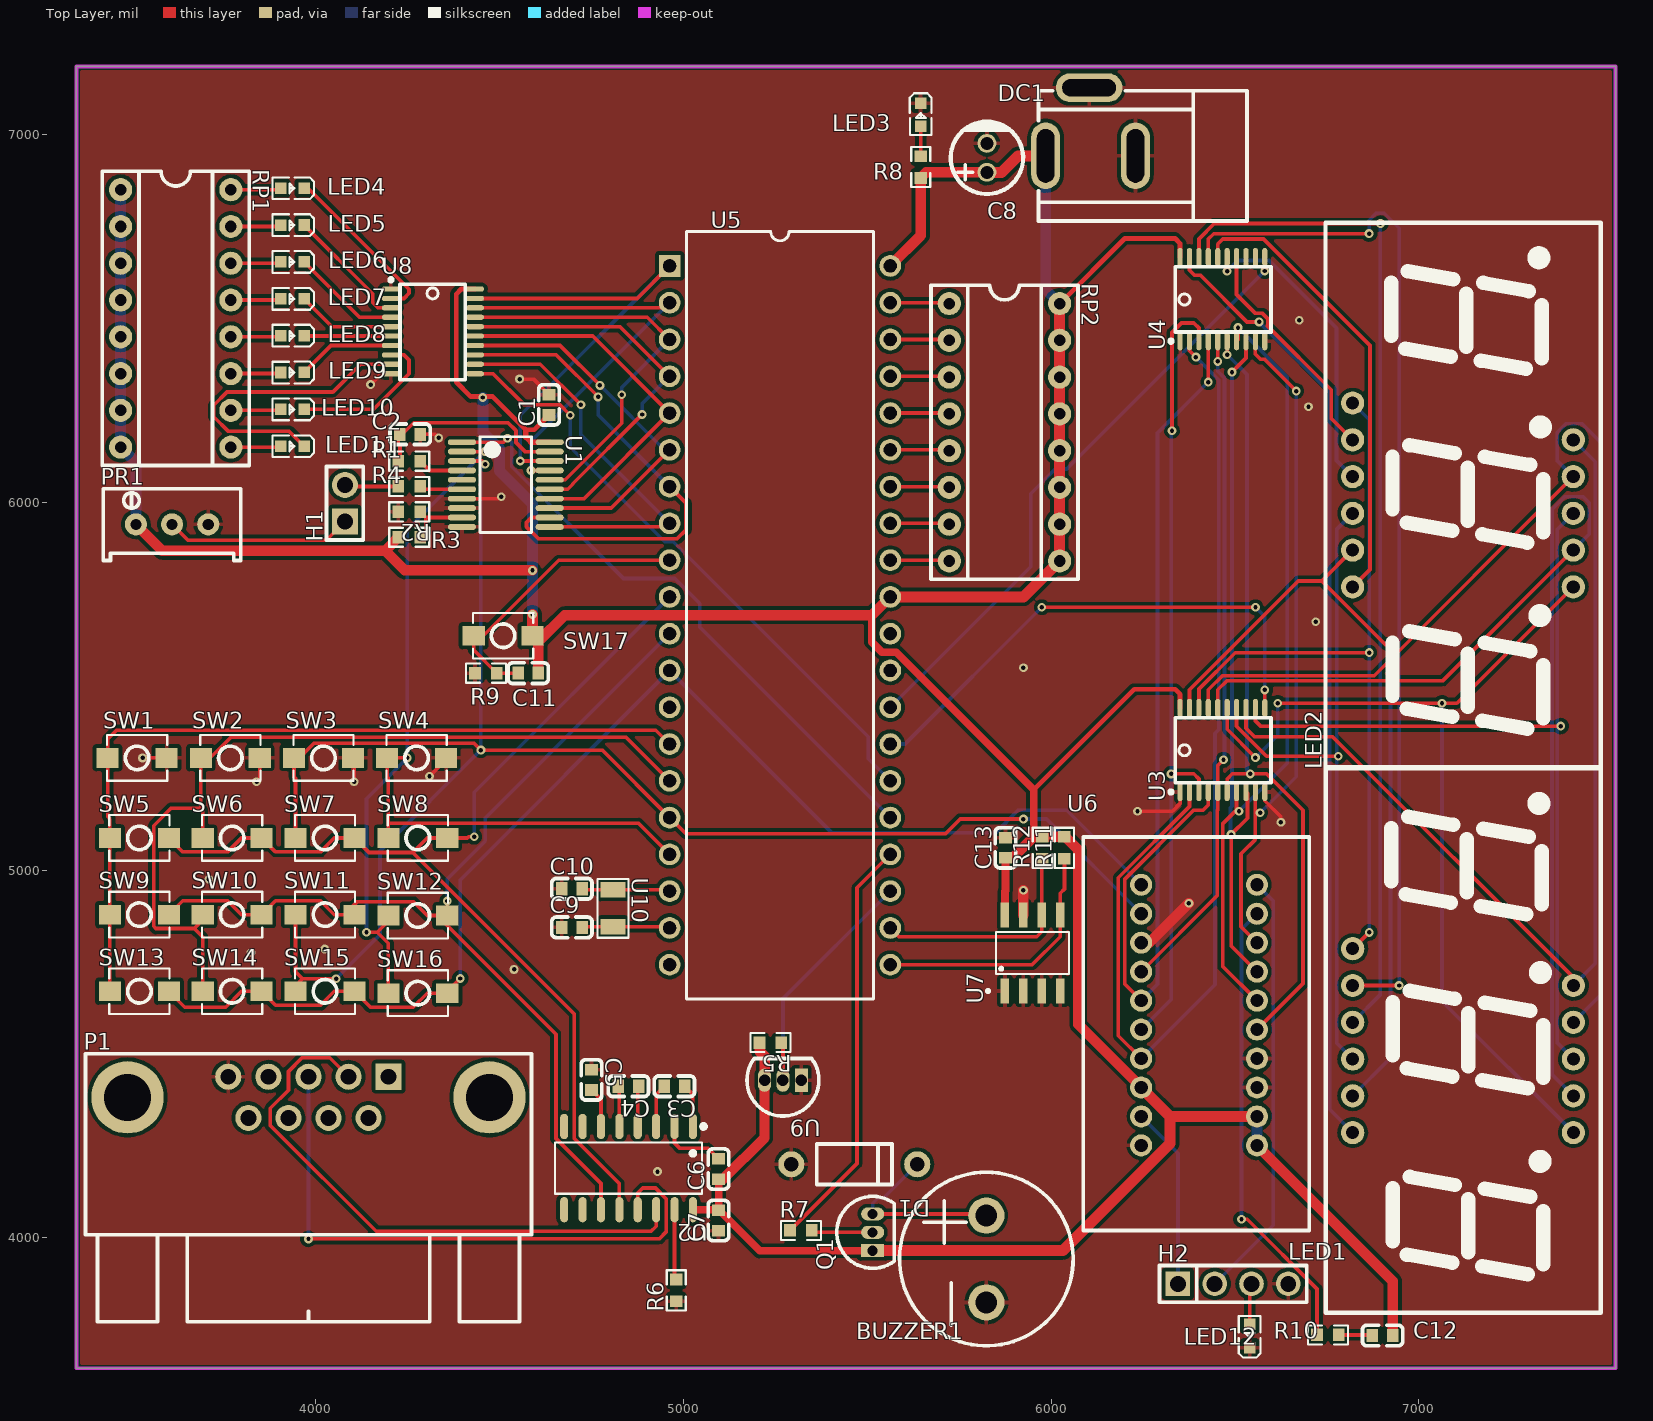
[diagram p0: Top Layer view]
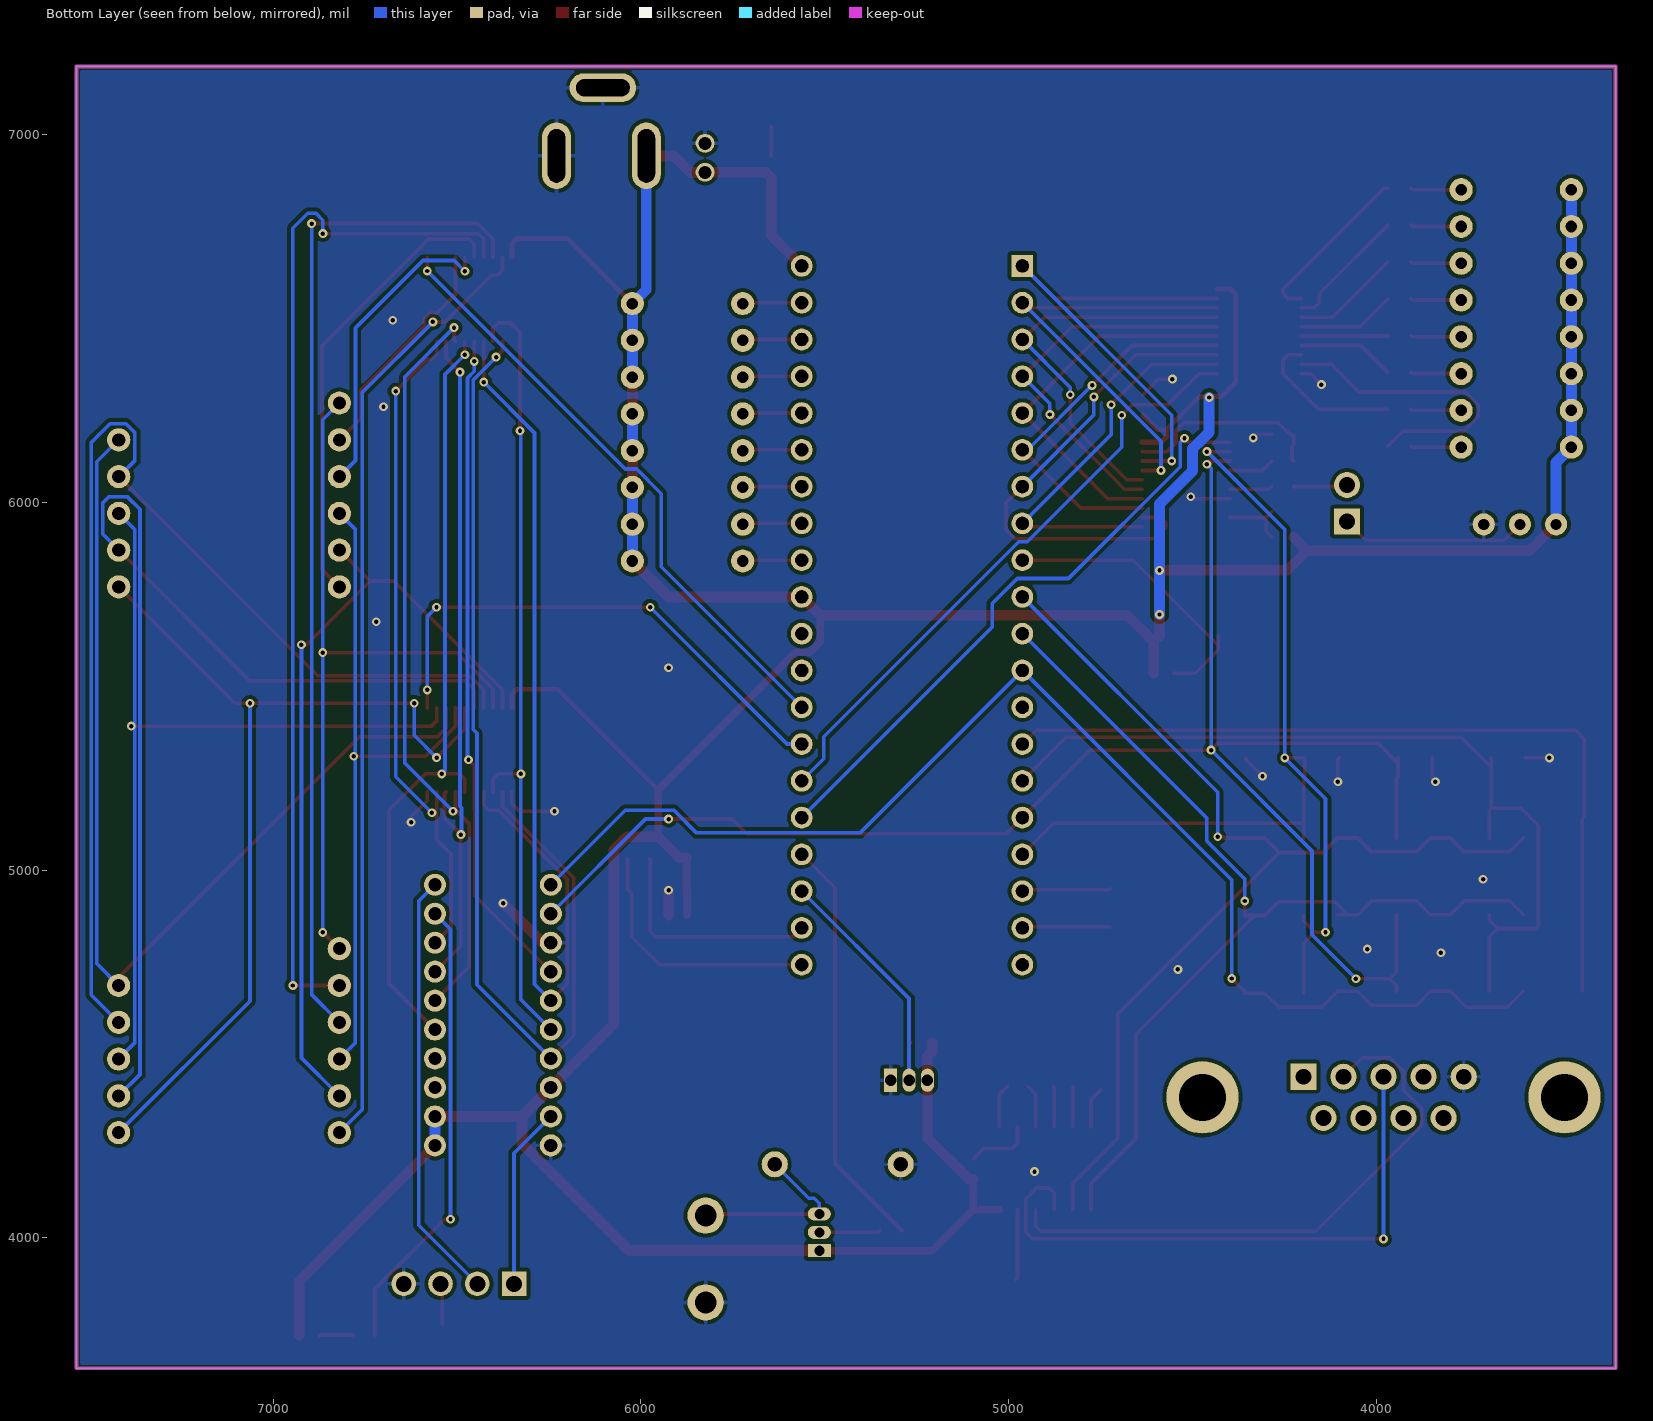
[diagram p1: Bottom Layer view, seen from below]
# Altium PCB MISC51981.pcbdoc
Units mil, origin at the board's own origin, x right, y up, seen from the top; angles counter-clockwise.
Board outline 4185 x 3540 mil, 2 copper layers (Top Layer, Bottom Layer), stack 62.206 mil thick; 74 components, 100 nets, 357 pads, 76 vias.

## Layer stack, top to bottom
Top Solder Mask Layer: solder mask 0.394, Dk 3.3
Top Layer: signal copper 1.379
Dielectric1: surface 59.449, FR4, Dk 4.5
Bottom Layer: signal copper 1.378
Bottom Solder Mask Layer: solder mask 0.394, Dk 3.3

## Board outline
3350,7185 3350,3645 7535,3645 7535,7185

## Design rules (kind name [scope] priority, off if disabled: settings)
BoardOutlineClearance copperThickness2oz_1 [All] p2 off: genericclearance=7.99 ignorepadtopadclearanceinfootprint=FALSE except(0: Arc-SplitContinuation Track-SplitContinuation SMDPad-SplitContinuation THPad-SplitContinuation Via-SplitContinuation Fill-SplitContinuation Region-SplitContinuation Poly-SplitContinuation Text-SplitContinuation Hole-SplitContinuation; 5.98: Arc-CutoutEdge SMDPad-CutoutEdge THPad-CutoutEdge Via-CutoutEdge Fill-CutoutEdge Region-CutoutEdge Text-CutoutEdge; 6.93: Hole-OutlineEdge Hole-CutoutEdge; 10: Poly-OutlineEdge Poly-CutoutEdge; 11.81: Arc-OutlineEdge Track-OutlineEdge SMDPad-OutlineEdge THPad-OutlineEdge Via-OutlineEdge Fill-OutlineEdge Region-OutlineEdge Text-OutlineEdge Track-CutoutEdge)
BoardOutlineClearance copperThickness1oz_1 [All] p4: genericclearance=4.02 ignorepadtopadclearanceinfootprint=FALSE except(0: Arc-SplitContinuation Track-SplitContinuation SMDPad-SplitContinuation THPad-SplitContinuation Via-SplitContinuation Fill-SplitContinuation Region-SplitContinuation Poly-SplitContinuation Text-SplitContinuation Hole-SplitContinuation; 6: SMDPad-CutoutEdge THPad-CutoutEdge Via-CutoutEdge Fill-CutoutEdge Region-CutoutEdge Text-CutoutEdge; 6.93: Hole-OutlineEdge Hole-CutoutEdge; 10: Poly-OutlineEdge Poly-CutoutEdge; 11.8: Arc-OutlineEdge Track-OutlineEdge SMDPad-OutlineEdge THPad-OutlineEdge Via-OutlineEdge Fill-OutlineEdge Region-OutlineEdge Text-OutlineEdge; 11.81: Arc-CutoutEdge Track-CutoutEdge)
Clearance copperThickness2oz [All] p1 off: gap=7.99 ignorepadtopadclearanceinfootprint=FALSE except(5.98: SMDPad-Track SMDPad-SMDPad THPad-Track SMDPad-THPad THPad-THPad Track-Via SMDPad-Via THPad-Via Via-Via Fill-Track Region-Track Fill-SMDPad Region-SMDPad Fill-THPad Region-THPad Fill-Via Region-Via Fill-Fill Fill-Region Region-Region Arc-Track Arc-SMDPad Arc-THPad Arc-Via Fill-Arc Region-Arc Arc-Arc Text-Track SMDPad-Text Text-THPad Text-Via Fill-Text Region-Text Arc-Text Text-Text; 6.93: Hole-Track Hole-SMDPad Hole-THPad Hole-Via Fill-Hole Region-Hole Hole-Arc Hole-Text; 10: Poly-Track Poly-SMDPad Poly-THPad Poly-Via Poly-Fill Poly-Region Poly-Poly Poly-Arc Poly-Text Poly-Hole)
Clearance copperThickness1oz [All] p3: gap=4.02 ignorepadtopadclearanceinfootprint=FALSE except(5.98: SMDPad-Track SMDPad-SMDPad THPad-Track SMDPad-THPad THPad-THPad Track-Via SMDPad-Via THPad-Via Via-Via Fill-Track Region-Track Fill-SMDPad Region-SMDPad Fill-THPad Region-THPad Fill-Via Region-Via Fill-Fill Fill-Region Region-Region; 6: Arc-Track Arc-SMDPad Arc-THPad Arc-Via Fill-Arc Region-Arc Arc-Arc Text-Track SMDPad-Text Text-THPad Text-Via Fill-Text Region-Text Arc-Text Text-Text; 6.93: Hole-Track Hole-SMDPad Hole-THPad Hole-Via Fill-Hole Region-Hole Hole-Arc Hole-Text; 10: Poly-Track Poly-SMDPad Poly-THPad Poly-Via Poly-Fill Poly-Region Poly-Poly Poly-Arc Poly-Text Poly-Hole)
Creepage creepage [All] p1: checkdistance=0 ignoreinternallayers=TRUE applytopolygonpour=TRUE
DiffPairsRouting differentialPair [All] p1: maxlimit=6 minlimit=6 mostfreqgap=6 toplayer_minwidth=5 toplayer_prefwidth=10 toplayer_maxwidth=100 toplayer_mingap=6 toplayer_prefgap=6 toplayer_maxgap=6 bottomlayer_minwidth=5 bottomlayer_prefwidth=10 bottomlayer_maxwidth=100 bottomlayer_mingap=6 bottomlayer_prefgap=6 bottomlayer_maxgap=6 maxuncoupledlength=10
HoleToHoleClearance otherClearance [All] p1: gap=11.81 allowstackedmicrovias=TRUE
Length netLength [All] p1: minlimit=0 maxlimit=0
MatchedLengths netLengthTolerance [All] p1: tolerance=1000
PasteMaskExpansion pasteMaskExpansion [All] p1: expansion=0
PlaneConnect innerPlane [All] p1: planeconnectstyle=Relief reliefexpansion=20 reliefentries=4 reliefconductorwidth=10 reliefairgap=10
PolygonConnect copperRegion [All] p1: connectstyle=Relief reliefconductorwidth=10 reliefentries=4 polygonreliefangle="90 Angle" airgapwidth=10 via.connectstyle=Relief via.reliefconductorwidth=10 via.reliefentries=4 via.polygonreliefangle="90 Angle" via.airgapwidth=10
RoutingVias viaSize [All] p1: holewidth=12.01 width=24.02 viastyle="Through Hole" minholewidth=11.81 minwidth=19.68 maxholewidth=248.03 maxwidth=393.7
SolderMaskExpansion solderMaskExpansion [IsVia] p1: expansion=-1000 istentingtop=TRUE
SolderMaskExpansion solderMaskExpansion [All] p2: expansion=2 istentingtop=FALSE
Width copperThickness2oz_2 [All] p1 off: maxlimit=100 minlimit=8 preferedwidth=10
Width PWR [(InNet('VCC'))] p2: maxlimit=10 minlimit=10 preferedwidth=10 toplayer_minwidth=10 toplayer_maxwidth=100 toplayer_prefwidth=30 bottomlayer_minwidth=10 bottomlayer_maxwidth=100 bottomlayer_prefwidth=30
Width copperThickness1oz_2 [All] p3: maxlimit=10 minlimit=10 preferedwidth=10 toplayer_minwidth=10 toplayer_maxwidth=100 toplayer_prefwidth=10 bottomlayer_minwidth=10 bottomlayer_maxwidth=100 bottomlayer_prefwidth=10

## Components (designator, comment, footprint, x,y, rotation, side; value= is the part's Value field where it differs from the comment)
BUZZER1 "buzzer" BUZ-TH_BD12.0-P6.00-D0.9-RD 5824.07,3942.5 r90 top
C1 "104" C0603 4635,6265 r90 top
C2 "104" C0603 4257.19,6185 r0 top
C3 "104" C0603 4975.96,4412.17 r180 top
C4 "104" C0603 4850.96,4412.17 r180 top
C5 "104" C0603 4750.56,4429.6 r270 top
C6 "104" C0603 5095.96,4187.17 r90 top
C7 "104" C0603 5095.96,4047.17 r90 top
C8 "100uF" CAP-TH_BD5.0-P2.00-D0.8-FD-10UF50VC110GL 5825.71,6936.62 r90 top
C9 "20PF" C0603 4697.26,4844.24 r0 top
C10 "20PF" C0603 4697.26,4949.24 r0 top
C11 "10uF" C0603 4578.45,5535.44 r0 top
C12 "104" C0603 6901.47,3734.39 r0 top
C13 "104" C0603 5876.39,5060.56 r90 top
D1 "" DO_1N4007 5465,4200 r180 top
DC1 "" DC-005_2.5 6112.46,6954.71 r0 top
H1 "" HDR-TH_2P-P2.54-V-M-1 4080,5997.34 r90 top
H2 "" HDR-TH_4P-P2.54-V-M 6495,3875 r0 top
LED1 "3631BS" LED-SEG-TH_11P-L37.5-W19.0-P2.54-LS15.2-BL_1 7120.32,4536.17 r90 top
LED2 "3631BS" LED-SEG-TH_11P-L37.5-W19.0-P2.54-LS15.2-BL_1 7120,6020 r90 top
LED3 "" LED_0603 5645.71,7051.62 r270 top
LED4 "" LED_0603 3935.58,6853.85 r180 top
LED5 "" LED_0603 3935.58,6753.63 r180 top
LED6 "" LED_0603 3935.58,6653.41 r180 top
LED7 "" LED_0603 3935.58,6553.19 r180 top
LED8 "" LED_0603 3935.58,6452.98 r180 top
LED9 "" LED_0603 3935.58,6352.76 r180 top
LED10 "" LED_0603 3935.58,6252.54 r180 top
LED11 "" LED_0603 3935.58,6152.32 r180 top
LED12 "" LED_0603 6540,3735 r90 top
P1 "DB9FL" DB9-TH_DB9F 3980.96,4382.17 r0 top
PR1 "10kΩ" R_3296 3610,5945 r0 top
Q1 "" S8550P_TO-92 5515,4015 r90 top
R1 "10K" R0603 4255,6112.04 r0 top
R2 "1K" R0603 4255,5974.01 r180 top
R3 "1K" R0603 4255,5905 r0 top
R4 "510K" R0603 4255,6043.03 r0 top
R5 "4.7K" R0603 5237.02,4531.02 r180 top
R6 "0" R0603 4980.96,3857.17 r90 top
R7 "2K" R0603 5320,4020 r0 top
R8 "1K" R0603 5645.71,6911.62 r270 top
R9 "10K" R0603 4463.45,5535.44 r0 top
R10 "0" R0603 6752.91,3736.03 r0 top
R11 "4.7K" R0603 6036.39,5060.56 r90 top
R12 "4.7K" R0603 5976.39,5060.56 r90 top
RP1 "" DIP-16_L20.3-W10.2-P2.54-LS7.6-BL 3620,6500 r270 top
RP2 "" DIP-16_L20.3-W10.2-P2.54-LS7.6-BL 5873.45,6190.44 r270 top
SW1 "" Key_SMD_3x4x2 3515,5305 r180 top
SW2 "" Key_SMD_3x4x2 3768.33,5305 r180 top
SW3 "" Key_SMD_3x4x2 4021.67,5305 r180 top
SW4 "" Key_SMD_3x4x2 4275,5305 r180 top
SW5 "" Key_SMD_3x4x2 3521.09,5087.32 r0 top
SW6 "" Key_SMD_3x4x2 3773.46,5087.32 r0 top
SW7 "" Key_SMD_3x4x2 4025.84,5087.32 r0 top
SW8 "" Key_SMD_3x4x2 4278.21,5087.32 r0 top
SW9 "" Key_SMD_3x4x2 3521.09,4878.83 r0 top
SW10 "" Key_SMD_3x4x2 3773.46,4878.83 r0 top
SW11 "" Key_SMD_3x4x2 4025.84,4878.83 r0 top
SW12 "" Key_SMD_3x4x2 4278.21,4876.33 r0 top
SW13 "" Key_SMD_3x4x2 3521.09,4670.34 r0 top
SW14 "" Key_SMD_3x4x2 3773.46,4670.34 r0 top
SW15 "" Key_SMD_3x4x2 4025.84,4670.34 r0 top
SW16 "" Key_SMD_3x4x2 4278.21,4665.34 r0 top
SW17 "" Key_SMD_3x4x2 4510.24,5637.16 r180 top
U1 "ADC0804CN" ADC0804CN 4529.5,6063.27 r270 top
U2 "MAX232ESE" MAX232ESE 5055.96,4302.17 r180 top
U3 "MC74HC573DW" MC74HC573DW 6350.95,5212.39 r90 top
U4 "MC74HC573DW" MC74HC573DW 6350.95,6438.19 r90 top
U5 "P89C51RC2HBP" P89C51RC23N_01 5218.38,5544.96 r270 top
U6 "DAC0832LCJ" DAC0832LCJ 6560,4960 r0 top
U7 "AT24C02" SOIC-8_L5.0-W4.0-P1.27-LS6.2-TL 5949.75,4774.49 r90 top
U8 "MC74HC573DW" MC74HC573DW 4205,6580 r0 top
U9 "DS18B20" TO-92-3_L4.9-W3.7-P1.27-L 5271.01,4428.68 r180 top
U10 "32768/10ppm/12.5pF" osc-smd_l3.2-w1.5 4808.9,4896.03 r270 top

## Footprints (in the part's own frame and the unit in brackets; to place one, negate y for a bottom-side part, rotate by r counter-clockwise, add the part's x,y. Pads: shape width x height; smd on the part's side, far side on the other; paste and mask are expansions set on the pad)
ADC0804CN [mm]
  oval 0.4x1.95 smd: 1(-2.544,-3.334) 2(-1.894,-3.334) 3(-1.244,-3.334) 4(-0.594,-3.334) 5(0.056,-3.334) 6(0.706,-3.334) 7(1.356,-3.334) 8(2.006,-3.334) 9(2.656,-3.334) 10(3.306,-3.334) 11(3.306,2.724) 12(2.656,2.724) 13(2.006,2.724) 14(1.356,2.724) 15(0.706,2.724) 16(0.056,2.724) 17(-0.594,2.724) 18(-1.244,2.724) 19(-1.894,2.724) 20(-2.544,2.724)
  silkscreen extent -2.92,-2.08 3.68,1.47
BUZ-TH_BD12.0-P6.00-D0.9-RD [mm]
  round 2.5 hole 1.5 paste+0 mask+0.05: 1(-3,0) 2(3,0)
  silkscreen extent -5.99,-5.99 5.99,5.99
C0603 [mm]
  rect 0.8x0.9 smd: 1(-0.7,0) 2(0.7,0)
  silkscreen extent -1.39,-0.71 1.39,0.71
CAP-TH_BD5.0-P2.00-D0.8-FD-10UF50VC110GL [mm]
  round 1.3 hole 0.9 paste+0 mask+0.051: 1(-1,0) 2(1,0)
  silkscreen extent -2.5,-2.5 2.5,2.5
DAC0832LCJ [mil]
  round 60 hole 36 paste+0 mask+2: 1(-314.96,0) 2(-314.96,-78.74) 3(-314.96,-157.48) 4(-314.96,-236.22) 5(-314.96,-314.96) 6(-314.96,-393.7) 7(-314.96,-472.44) 8(-314.96,-551.18) 9(-314.96,-629.92) 10(-314.96,-708.66) 11(0,0) 12(0,-78.74) 13(0,-157.48) 14(0,-236.22) 15(0,-314.96) 16(0,-393.7) 17(0,-472.44) 18(0,-551.18) 19(0,-629.92) 20(0,-708.66)
  silkscreen extent -472,-940 142,130
DB9-TH_DB9F [mm]
  rect 1.8x1.8 hole 1.1: 1(5.54,1.42)
  round 1.8 hole 1.1: 2(2.77,1.42) 3(0,1.42) 4(-2.77,1.42) 5(-5.54,1.42) 6(4.155,-1.42) 7(1.385,-1.42) 8(-1.385,-1.42) 9(-4.155,-1.42)
  round 5 hole 3.25: 10(-12.5,0) 11(12.5,0)
  silkscreen extent -15.4,-15.5 15.4,3
DC-005_2.5 [mm]
  oval 2x4.6 hole 1.2 slot 3.7 at 90 deg paste+0 mask+0.051: 1(-3.227,-0.318) 2(2.973,-0.318)
  oval 4.6x2 hole 1.2 slot 3.7 at 0 deg paste+0 mask+0.051: 3(-0.227,4.382)
  silkscreen extent -3.73,-4.82 10.67,4.18
DIP-16_L20.3-W10.2-P2.54-LS7.6-BL [mm]
  round 1.6 hole 0.8: 1(-8.89,-3.81) 2(-6.35,-3.81) 3(-3.81,-3.81) 4(-1.27,-3.81) 5(1.27,-3.81) 6(3.81,-3.81) 7(6.35,-3.81) 8(8.89,-3.81) 9(8.89,3.81) 10(6.35,3.81) 11(3.81,3.81) 12(1.27,3.81) 13(-1.27,3.81) 14(-3.81,3.81) 15(-6.35,3.81) 16(-8.89,3.81)
  silkscreen extent -10.16,-5.08 10.16,5.08
DO_1N4007 [mm]
  round 1.8 hole 1 paste+0 mask+0.051: 1(-4.35,0) 2(4.35,0)
  silkscreen extent -2.6,-1.4 2.6,1.4
HDR-TH_2P-P2.54-V-M-1 [mm]
  rect 1.8x1.8 hole 1.1: 1(-1.27,0)
  round 1.8 hole 1.1: 2(1.27,0)
  silkscreen extent -2.54,-1.27 2.54,1.27
HDR-TH_4P-P2.54-V-M [mm]
  rect 1.7x1.7 hole 1.1: 1(-3.81,0)
  round 1.7 hole 1.1: 2(-1.27,0) 3(1.27,0) 4(3.81,0)
  silkscreen extent -5.08,-1.27 5.08,1.27
Key_SMD_3x4x2 [mm]
  rect 1.53x1.36 smd paste+0 mask+0.051: 1(-2.035,0) 2(2.035,0)
  silkscreen extent -2.08,-1.58 2.08,1.58
LED-SEG-TH_11P-L37.5-W19.0-P2.54-LS15.2-BL_1 [mm]
  round 1.6 hole 0.9: 1(-6.35,-7.62) 2(-3.81,-7.62) 3(-1.27,-7.62) 4(1.27,-7.62) 5(3.81,-7.62) 7(6.35,7.62) 8(3.81,7.62) 9(1.27,7.62) 10(-1.27,7.62) 11(-3.81,7.62) 12(-6.35,7.62)
  silkscreen extent -18.8,-9.51 18.8,9.49
LED_0603 [mil]
  rect 31.5x31.5 smd paste+0 mask+2: 1(-33.5,-0.4) 2(29.5,-0.2)
  silkscreen extent -61,-30 53,30
MAX232ESE [mm]
  oval 0.56x1.745 smd paste+0.102 mask+0.051: 1(0.755,-0.016) 2(2.025,-0.016) 3(3.295,-0.016) 4(4.565,-0.016) 5(5.835,-0.016) 6(7.105,-0.016) 7(8.375,-0.016) 8(9.645,-0.016) 9(9.645,5.728) 10(8.375,5.728) 11(7.105,5.728) 12(5.835,5.728) 13(4.565,5.728) 14(3.295,5.728) 15(2.025,5.728) 16(0.755,5.728)
  silkscreen extent -0.13,-0.17 10.28,4.63
MC74HC573DW [mm]
  oval 1.26x0.36 smd: 1(0,0) 2(0,-0.65) 3(0,-1.3) 4(0,-1.95) 5(0,-2.6) 6(0,-3.25) 7(0,-3.9) 8(0,-4.55) 9(0,-5.2) 10(0,-5.85) 11(5.8,-5.85) 12(5.8,-5.2) 13(5.8,-4.55) 14(5.8,-3.9) 15(5.8,-3.25) 16(5.8,-2.6) 17(5.8,-1.95) 18(5.8,-1.3) 19(5.8,-0.65) 20(5.8,0)
  silkscreen extent -0.05,-6.27 5.13,0.68
osc-smd_l3.2-w1.5 [mm]
  rect 1.05x1.7 smd: 1(-1.275,0) 2(1.275,0)
  silkscreen extent -2.03,-1.08 2.03,1.08
P89C51RC23N_01 [mm]
  rect 1.5x1.5 hole 0.9 slot 0.905 at 90 deg paste+0 mask+0.051: 1(-27.883,-6.489)
  round 1.5 hole 0.9 slot 0.905 at 90 deg paste+0 mask+0.051: 2(-25.343,-6.489) 3(-22.803,-6.489) 4(-20.263,-6.489) 5(-17.723,-6.489) 6(-15.183,-6.489) 7(-12.643,-6.489) 8(-10.103,-6.489) 9(-7.563,-6.489) 10(-5.023,-6.489) 11(-2.483,-6.489) 12(0.057,-6.489) 13(2.597,-6.489) 14(5.137,-6.489) 15(7.677,-6.489) 16(10.217,-6.489) 17(12.757,-6.489) 18(15.297,-6.489) 19(17.837,-6.489) 20(20.377,-6.489) 21(20.377,8.751) 22(17.837,8.751) 23(15.297,8.751) 24(12.757,8.751) 25(10.217,8.751) 26(7.677,8.751) 27(5.137,8.751) 28(2.597,8.751) 29(0.057,8.751) 30(-2.483,8.751) 31(-5.023,8.751) 32(-7.563,8.751) 33(-10.103,8.751) 34(-12.643,8.751) 35(-15.183,8.751) 36(-17.723,8.751) 37(-20.263,8.751) 38(-22.803,8.751) 39(-25.343,8.751) 40(-27.883,8.751)
  silkscreen extent -30.25,-5.32 22.75,7.58
R0603 [mil]
  rect 31.75x34.02 smd paste-3937.01 mask+2: 1(-29.66,0) 2(29.66,0)
  silkscreen extent -55,-26 55,26
R_3296 [mil]
  round 60 hole 30 paste+0 mask+2: 1(-98.4,-5) 2(0,-5) 3(98.4,-5)
  silkscreen extent -187,-103 187,92
S8550P_TO-92 [mm]
  rect 0.9x1.6 hole 0.7 paste+0 mask+0.051: 1(-1.27,0)
  oval 0.9x1.6 hole 0.7 paste+0 mask+0.051: 2(0,0) 3(1.27,0)
  silkscreen extent -2.48,-1.5 2.48,2.48
SOIC-8_L5.0-W4.0-P1.27-LS6.2-TL [mil]
  rect 68.92x23.18 smd: 1(-103.36,75) 2(-103.36,25) 3(-103.36,-25) 4(-103.36,-75) 5(103.36,-75) 6(103.36,-25) 7(103.36,25) 8(103.36,75)
  silkscreen extent -107,-99 57,125
TO-92-3_L4.9-W3.7-P1.27-L [mm]
  rect 0.9x1.6 hole 0.8: 1(-1.27,0)
  oval 0.9x1.6 hole 0.8: 2(0,0) 3(1.27,0)
  silkscreen extent -2.48,-1.5 2.48,2.48

## Via types
v1: diameter 24.02, hole 12, Top Layer to Bottom Layer, 76 vias

## Nets (pads, with @x,y where several pads share a name; then routed paths per layer and width w, separated by ;. In a path a pad name is that pad's centre, name@x,y a point inside that pad or via, vN(x,y) a via of type N, cw(c..) or ccw(c..) an arc to the next point about the centre after c; other vN are vias at no path point)
18B20: R5.1 U5.23 U9.2 | length 739.1
  Top Layer w10: R5.1 5271.01,4526.69 U9.2
  Bottom Layer w10: U9.2 5271.01,4650.81 U5.23
$1N14: R1.2 U1.4 | length 124.1
  Top Layer w10: R1.2 4310.04,6086.66 U1.4@4398.25,6086.66
$1N15: C2.1 R1.1 U1.19 | length 558.8
  Top Layer w10: R1.1 4229.93,6116.63 4229.93,6151.61 4225.34,6156.2 C2.1@4225.34,6174.83 ; C2.1 4225.34,6180.71 C2.1@4225.34,6174.83 ; U1.19@4636.75,6137.84 4569.86,6137.84 4545,6162.7 4545,6195 4523.4,6216.6 4267.11,6216.6 C2.1@4225.34,6174.83
$1N18: H1.1 PR1.2 | length 509
  Top Layer w10: PR1.2 3653.36,5896.64 4029.3,5896.64 H1.1
$1N20: R2.1 R3.2 U1.9 | length 180
  Top Layer w10: R3.2 4299.98,5920.32 R2.1@4299.98,5958.7 ; R2.1 R2.1@4299.98,5958.7 ; U1.9@4398.25,5958.7 R2.1@4299.98,5958.7
$1N23: R4.2 U1.6 | length 116.7
  Top Layer w10: R4.2 4292.22,6035.47 U1.6@4398.25,6035.47
$1N24: H1.2 R4.1 | length 147.1
  Top Layer w10: H1.2 4084.31,6043.03 R4.1
$1N28: C3.1 U2.1 | length 118.8
  Top Layer w10: C3.1 5026.22,4389.46 U2.1
$1N29: C3.2 U2.3 | length 118.5
  Top Layer w10: U2.3 4926.22,4389.98 C3.2
$1N30: C4.2 U2.5 | length 110.5
  Top Layer w10: C4.2 4826.22,4409.34 U2.5
$1N31: C4.1 U2.4 | length 110.3
  Top Layer w10: U2.4 4876.22,4409.86 C4.1
$1N34: R6.2 U2.15 | length 191.8
  Top Layer w10: U2.15 4976.22,3891.56 R6.2
$1N36: P1.3 U2.13 | length 1651.5
  Top Layer w10: v1(3980.96,3997.14) 4934.41,3997.14 4953.36,4016.09 4953.36,4106.56 4924.44,4135.48 4889.99,4135.48 4876.22,4121.71 U2.13
  Bottom Layer w10: v1(3980.96,3997.14) P1.3
$1N37: P1.2 U2.14 | length 1586.6
  Top Layer w10: P1.2 4038.48,4489.61 3963.45,4489.61 3926.43,4452.59 3926.43,4401.4 3877.24,4352.21 3877.24,4305.64 4165.1,4017.78 4912.45,4017.78 4926.22,4031.55 U2.14
$1N38: C5.2 U2.6 | length 109.9
  Top Layer w10: C5.2 4776.22,4376.38 U2.6
$1N40: C6.2 U2.2 | length 182.6
  Top Layer w10: U2.2 4976.22,4257.73 4989.99,4243.96 5066.72,4243.96 C6.2
$1N109: BUZZER1.2 D1.1 Q1.3 | length 505
  Top Layer w10: Q1.3 5819.68,4065 BUZZER1.2
  Bottom Layer w10: Q1.3 5515,4093.95 5528.77,4107.72 5543.98,4107.72 D1.1
$1N111: Q1.2 R7.2 | length 167.4
  Top Layer w10: R7.2 5354.66,4015 Q1.2
$1N114: LED3.2 R8.1 | length 80.9
  Top Layer w10: LED3.2 5645.51,6941.48 R8.1
$1N128: LED4.1 U8.2 | length 465.3
  Top Layer w10: LED4.1@3969.08,6854.25 3979.44,6854.25 4254.3,6579.39 4254.3,6568.18 4240.53,6554.41 U8.2
$1N129: LED5.1 U8.3 | length 343.7
  Top Layer w10: LED5.1 4155.7,6567.41 4155.7,6542.59 4169.47,6528.82 U8.3
$1N130: LED5.2 RP1.15 | length 137.7
  Top Layer w10: RP1.15 3902.25,6750 LED5.2
$1N131: LED7.2 RP1.13 | length 137.5
  Top Layer w10: RP1.13 3902.68,6550 LED7.2
$1N132: LED7.1 U8.5 | length 267.4
  Top Layer w10: LED7.1 4045.04,6477.64 U8.5
$1N133: LED6.1 U8.4 | length 298.3
  Top Layer w10: LED6.1 4119.67,6503.23 U8.4
$1N134: LED9.2 RP1.11 | length 137.3
  Top Layer w10: RP1.11 3903.12,6350 LED9.2
$1N135: LED9.1 U8.7 | length 266.3
  Top Layer w10: LED9.1 4042.38,6426.46 U8.7
$1N136: LED8.1 U8.6 | length 236.5
  Top Layer w10: LED8.1 3970.41,6452.05 U8.6
$1N137: LED11.2 RP1.9 | length 137.1
  Top Layer w10: RP1.9 3903.56,6150 LED11.2
$1N138: LED11.1 U8.9 | length 837.8
  Top Layer w10: LED11.1 3928.94,6192.86 3763.36,6192.86 3723.25,6232.97 3723.25,6263.68 3759.57,6300 4047.27,6300 4122.55,6375.28 U8.9
$1N139: LED10.1 U8.8 | length 417.9
  Top Layer w10: LED10.1 4157.9,6252.94 4254.3,6349.34 4254.3,6387.1 4240.53,6400.87 U8.8
$1N140: LED4.2 RP1.16 | length 137.8
  Top Layer w10: RP1.16 3902.03,6850 LED4.2@3906.08,6854.05
$1N141: LED6.2 RP1.14 | length 137.6
  Top Layer w10: RP1.14 3902.46,6650 LED6.2
$1N142: LED8.2 RP1.12 | length 137.4
  Top Layer w10: RP1.12 3902.9,6450 LED8.2
$1N143: LED10.2 RP1.10 | length 137.2
  Top Layer w10: RP1.10 3903.34,6250 LED10.2
$1N162: RP2.8 U5.32 | length 161.5
  Top Layer w10: U5.32 5721.17,5842.72 RP2.8
$1N163: RP2.7 U5.33 | length 161.5
  Top Layer w10: U5.33 5721.17,5942.72 RP2.7
$1N164: RP2.6 U5.34 | length 161.5
  Top Layer w10: U5.34 5721.17,6042.72 RP2.6
$1N165: RP2.5 U5.35 | length 161.5
  Top Layer w10: U5.35 5721.17,6142.72 RP2.5
$1N166: RP2.4 U5.36 | length 161.5
  Top Layer w10: U5.36 5721.17,6242.72 RP2.4
$1N167: RP2.3 U5.37 | length 161.5
  Top Layer w10: U5.37 5721.17,6342.72 RP2.3
$1N168: RP2.2 U5.38 | length 161.5
  Top Layer w10: U5.38 5721.17,6442.72 RP2.2
$1N169: RP2.1 U5.39 | length 161.5
  Top Layer w10: U5.39 5721.17,6542.72 RP2.1
$1N205: C12.1 R10.2 | length 92
  Top Layer w10: R10.2 6872.27,3736.03 C12.1
$1N206: R10.1 U6.12 | length 1256.9
  Top Layer w10: v1(6517.84,4050.78) 6533.49,4050.78 6723.24,3861.03 R10.1
  Bottom Layer w10: v1(6517.84,4050.78) 6517.84,4839.1 U6.12
$1N207: H2.2 U6.11 | length 1169.3
  Bottom Layer w10: H2.2 6604.28,4034.28 6604.28,4915.72 U6.11
$1N208: H2.1 U6.9 | length 496.5
  Bottom Layer w10: U6.9 6345.01,4230.12 H2.1
$1N209: H2.3 LED12.2 | length 112.5
  Top Layer w10: LED12.2 6540.2,3870.2 H2.3
A: LED1.11 LED2.11 U3.19 | length 2178.1
  Top Layer w10: U3.19 6376.53,5490.04 6672.53,5786.04 6736.03,5786.04 ; LED2.11 6736.04,5786.03 ; v1(6923.17,5612.46) 6909.61,5612.46 6736.04,5786.03
  Bottom Layer w10: LED1.11 6923.17,4489.01 v1(6923.17,5612.46)
ALE: U5.30
B: LED1.7 LED2.7 U3.18 | length 2077.1
  Top Layer w10: U3.18 6402.12,5492.23 6501.07,5591.18 v1(6865.21,5591.18) ; LED1.7 6864.63,4830.47 v1(6865.21,4830.47)
  Bottom Layer w10: LED2.7 6865.21,6224.79 v1(6865.21,5591.18) v1(6865.21,4830.47)
C: LED1.4 LED2.4 U3.17 | length 3176.8
  Top Layer w10: U3.17 6427.71,5490.04 6466.24,5528.57 6878.57,5528.57 LED2.4
  Bottom Layer w10: LED2.4 7376.09,6113.91 7376.09,6189.46 7400.39,6213.76 7443.82,6213.76 7494.72,6162.86 7494.72,4660.56 LED1.4
CSAD: U1.1 U5.25 | length 1672
  Top Layer w10: U1.1@4398.25,6163.43 4511.43,6163.43 v1(4522.01,6174.01)
  Bottom Layer w10: v1(4522.01,6174.01) 4533.6,6162.41 4533.6,6096.75 4837.63,5792.72 4976.54,5792.72 5044.7,5724.56 5044.7,5660.93 U5.25
D: LED1.2 LED2.2 U3.16 | length 3060.3
  Top Layer w10: U3.16 6453.3,5490.04 6477.63,5514.37 7064.37,5514.37 LED2.2
  Bottom Layer w10: LED2.2 7463.07,5913.07 7463.07,5999.06 7447.37,6014.76 7396.18,6014.76 7362.4,5980.98 7362.4,4444.08 LED1.2
D0: U3.2 U4.2 U6.7 | length 2901.5
  Top Layer w10: U6.7 6183.03,4549.58 6183.03,4979.25 6376.53,5172.76 U3.2 ; U4.2 6376.53,6412.22 v1(6393.85,6394.91)
  Bottom Layer w10: U6.7 6445.74,4688.26 6445.74,5371.86 6455.9,5382.02 6455.9,6332.85 v1(6393.85,6394.91)
D1: U3.3 U4.3 U6.6 | length 2172
  Top Layer w10: v1(6326.63,5261.69) 6388.35,5261.69 6402.12,5247.92 U3.3 ; v1(6328.92,6194.66) 6328.92,6461.77 6354.64,6487.49 6388.35,6487.49 6402.12,6473.72 U4.3
  Bottom Layer w10: U6.6 6326.63,4647.88 v1(6326.63,5261.69) 6326.63,6192.37 v1(6328.92,6194.66)
D2: U3.4 U4.4 U6.5 | length 2563.5
  Top Layer w10: U6.5 6200.84,4689.25 6200.84,4975.63 6388.3,5163.09 6413.94,5163.09 6427.71,5176.86 U3.4 ; v1(6427.71,6326.93) U4.4
  Bottom Layer w10: U6.5 6289.56,4689.55 6289.56,6188.77 v1(6427.71,6326.93)
D3: U3.5 U4.5 U6.4 | length 1815.9
  Top Layer w10: U6.4 6452.29,4931.03 6452.29,5162.08 6453.3,5163.09 U3.5 6453.3,5284.27 v1(6468.9,5299.87) ; v1(6453.3,6383) U4.5
  Bottom Layer w10: v1(6453.3,6383) 6453.3,6356.11 6471.72,6337.69 6471.72,5302.69 v1(6468.9,5299.87)
D4: U3.6 U4.6 U6.16 | length 2139.2
  Top Layer w10: U3.6 6478.89,5247.92 6492.66,5261.69 v1(6541.74,5261.69) 6586.2,5261.69 6685,5162.9 6685,4691.3 U6.16 ; v1(6478.89,6401.11) U4.6
  Bottom Layer w10: v1(6478.89,6401.11) 6532.64,6347.36 6532.64,5270.79 v1(6541.74,5261.69)
D5: U3.7 U4.7 U6.15 | length 2093.3
  Top Layer w10: U3.7 v1@6504.48,5163.09 ; U4.7 6508.32,6442.03 v1(6508.32,6475.16) ; v1(6511.07,5159.8) 6507.77,5159.8 v1@6504.48,5163.09 ; U6.15 6466.48,4738.56 6466.48,5125.09 v1@6504.48,5163.09
  Bottom Layer w10: v1(6508.32,6475.16) 6641.95,6341.53 6641.95,5290.68 v1(6511.07,5159.8)
D6: U3.8 U4.8 U6.14 | length 1897.7
  Top Layer w10: v1(6492.06,6354.16) 6530.07,6392.16 U4.8 ; U3.8 6534.23,5208.23 6534.23,5141.19 v1(6489.64,5096.6) 6489.64,4794.14 U6.14
  Bottom Layer w10: v1(6489.64,5096.6) 6487.91,5098.33 6487.91,5169.38 6492.06,5173.53 v1(6492.06,6354.16)
D7: U3.9 U4.9 U6.13 | length 1832.3
  Top Layer w10: U3.9 6555.66,5155.91 ; U4.9 6555.66,6402.66 6569.43,6388.89 6580.22,6388.89 v1(6666.72,6302.39) ; U6.13 6516.42,4846.1 6516.42,5044.15 6555.66,5083.39 6555.66,5155.91 ; v1(6568.57,5155.91) 6555.66,5155.91
  Bottom Layer w10: v1(6568.57,5155.91) 6666.72,5254.06 v1(6666.72,6302.39)
DB1: U1.18 U5.1 U8.19 | length 1344.8
  Top Layer w10: U8.19@4433.35,6554.41 4874.6,6554.41 U5.1 ; v1(4556.77,6112.25) U1.18@4636.75,6112.25
  Bottom Layer w10: v1(4556.77,6112.25) 4556.77,6236.58 U5.1
DB2: U1.17 U5.2 U8.18 | length 1198.2
  Top Layer w10: U8.18@4433.35,6528.82 4949.01,6528.82 U5.2 ; v1(4586.02,6086.66) U1.17@4636.75,6086.66
  Bottom Layer w10: v1(4586.02,6086.66) 4586.02,6165.83 U5.2
DB3: U1.16 U5.3 U8.17 | length 1096
  Top Layer w10: U8.17@4433.35,6503.23 4902.4,6503.23 U5.3 ; U1.16@4636.75,6061.07 4678.85,6061.07 4832.59,6214.81 v1(4832.59,6292.33)
  Bottom Layer w10: v1(4832.59,6292.33) 4832.59,6312.4 U5.3
DB4: U1.15 U5.4 U8.16 | length 1056.6
  Top Layer w10: U8.16@4433.35,6477.64 4827.99,6477.64 U5.4 ; U1.15@4636.75,6035.47 4685.87,6035.47 4699.64,6049.24 4699.64,6050.37 v1(4888.1,6238.83)
  Bottom Layer w10: v1(4888.1,6238.83) 4888.1,6267.91 U5.4
DB5: U1.14 U5.5 U8.15 | length 1038.9
  Top Layer w10: U8.15@4433.35,6452.05 4753.58,6452.05 U5.5 4730.07,6009.88 U1.14@4636.75,6009.88
DB6: U1.13 U5.6 U8.14 | length 1038.9
  Top Layer w10: U8.14@4433.35,6426.46 4664.83,6426.46 v1(4773.32,6317.97) ; U1.13@4636.75,5984.29 4804.48,5984.29 U5.6
  Bottom Layer w10: v1(4773.32,6317.97) 4948.57,6142.72 U5.6
DB7: U1.12 U5.7 U8.13 | length 1380.6
  Top Layer w10: U8.13@4433.35,6400.87 4654.37,6400.87 v1(4768.55,6286.69) ; U1.12@4636.75,5958.7 4587.64,5958.7 4573.87,5944.93 4573.87,5933.1 4606.27,5900.7 4983.22,5900.7 5007.36,5924.84 5007.36,5998.27 U5.7
  Bottom Layer w10: v1(4768.55,6286.69) 4768.55,6237.08 U5.7
DB8: U1.11 U5.8 U8.12 | length 1086.3
  Top Layer w10: U8.12@4433.35,6375.28 4611.38,6375.28 v1(4721.61,6265.05) ; U1.11@4636.75,5933.11 4953.3,5933.11 U5.8
  Bottom Layer w10: v1(4721.61,6265.05) 4721.61,6184.02 U5.8
DIOLA: U5.26 U8.11 | length 1673.9
  Top Layer w10: U8.11@4433.35,6349.68 4482.65,6349.68 4566.67,6265.66 4663.87,6265.66 v1(4692.76,6236.77)
  Bottom Layer w10: v1(4692.76,6236.77) 4692.76,6149.89 4949.93,5892.72 4972.63,5892.72 5503.03,5362.32 5503.03,5302.6 U5.26
DP: LED1.3 LED2.3 U3.12 | length 2400.1
  Top Layer w10: U3.12 6555.66,5405.2 6569.43,5391.43 v1(7385.8,5391.43)
  Bottom Layer w10: v1(7385.8,5391.43) v1@7376.8,5391.43 ; LED2.3 7376.8,5926.8 v1@7376.8,5391.43 ; LED1.3 7376.8,4529.68 v1@7376.8,5391.43
DULA: U3.11 U5.27 | length 1431.6
  Top Layer w10: v1(5974.9,5714.71) v1(6555.99,5714.71) ; U3.11 v1(6581.26,5490.04)
  Bottom Layer w10: U5.27 5602.91,5342.72 v1(5974.9,5714.71) ; v1(6555.99,5714.71) 6581.26,5689.44 v1(6581.26,5490.04)
E: LED1.1 LED2.1 U3.15 | length 2589.9
  Top Layer w10: U3.15 6478.89,5382.58 v1(6555.8,5305.67) ; v1(6616.52,5453.57) v1(7063.17,5453.57) 7103.57,5453.57 LED2.1
  Bottom Layer w10: v1(6555.8,5305.67) 6616.52,5366.39 v1(6616.52,5453.57) ; v1(7063.17,5453.57) 7063.17,4643.31 LED1.1
F: LED1.10 LED2.10 U3.14 | length 1882.5
  Top Layer w10: U3.14 6504.48,5391.33 6586.16,5309.65 v1(6780.82,5309.65)
  Bottom Layer w10: v1(6780.82,5309.65) v1@6777.28,5309.65 ; LED2.10 6777.28,5927.28 v1@6777.28,5309.65 ; LED1.10 6777.28,4529.2 v1@6777.28,5309.65
G: LED1.5 LED2.5 U3.13 | length 2781
  Top Layer w10: U3.13 6530.07,5385.81 6553.21,5362.67 6765.48,5362.67 7420.32,4707.83 LED1.5
  Bottom Layer w10: LED2.5 7479.89,6110.11 7479.89,4745.73 LED1.5
GND: BUZZER1.1 C1.2 C2.2 C5.1 C7.1 C8.2 C9.1 C10.1 C13.2 D1.2 DC1.2 DC1.3 H2.4 LED3.1 LED12.1 P1.5 PR1.3 R2.2 R6.1 R9.1 SW1.1 SW2.1 SW3.1 SW4.1 U1.7 U1.8 U1.10 U3.1 U3.10 U4.1 U4.10 U6.3 U6.10 U6.17 U6.18 U7.1 U7.2 U7.3 U7.4 U7.7 U8.1 U8.10 U9.1 | length 1095.1
  Top Layer w10: v1(3530,5305) SW1.1 ; v1(3840,5240) 3848.45,5248.45 SW2.1 ; SW3.1 4105,5301.79 v1(4105,5240) ; v1(4150,6320) 4179.69,6349.69 U8.10 ; C2.2 4325,6185 v1(4335,6175) ; v1(4310,5255) 4355.12,5300.12 SW4.1 ; U1.7 4499.88,6009.88 v1(4505,6015) ; v1(4555,6335) 4592.56,6335 C1.2 ; v1(6235,5160) 6330,5160 6350.95,5180.95 U3.1 ; U3.10 6581.26,5188.74 6625,5145 v1(6625,5130)
  Top Layer w28.56: U7.7 5925,4878.1 v1(5925,4945) ; U6.3 6267.52,4802.52 v1(6375,4910)
  other v1: 4930,4180 4540,4730 3825,4775 4025,4785 3710,4975 5925,5550 6720,5675 6700,6260 6675,6495
INT0: SW13.2 SW14.2 SW15.2 SW16.2 U5.12 U6.1 | length 3561.8
  Top Layer w10: SW13.2 3644.28,4627.26 3755.88,4627.26 3798.96,4670.34 SW14.2 3891.5,4632.42 4013.41,4632.42 4051.33,4670.34 SW15.2 4148.87,4627.42 4265.79,4627.42 4303.71,4665.34 SW16.2@4353.61,4665.34 ; SW16.2 SW16.2@4353.61,4665.34 ; v1(4393.52,4705.25) SW16.2@4353.61,4665.34
  Bottom Layer w10: v1(4393.52,4705.25) 4393.52,4973.33 U5.12 5404.56,5101.07 5849.01,5101.07 5910.32,5162.38 6042.67,5162.38 U6.1
INT1: U5.13
LCDEN: SW1.2 SW5.1 SW9.1 SW13.1 U5.14 | length 2242.1
  Top Layer w10: SW13.1 SW9.1 SW5.1 3440.96,5138.59 3434.88,5144.67 SW1.2 3434.88,5356.27 3459.06,5380.45 4925.18,5380.45 U5.14
M11: LED1.12 U4.19 | length 2592.7
  Top Layer w10: U4.19 6376.53,6631 6390.31,6617.23 6406.32,6617.23 6533.07,6490.48 v1(6565.68,6490.48)
  Bottom Layer w10: v1(6565.68,6490.48) 6757.66,6298.5 6757.66,4348.82 LED1.12
M12: LED1.9 U4.18 | length 2763.2
  Top Layer w10: U4.18 6402.12,6715.9 6444.14,6757.92 v1(6895.6,6757.92)
  Bottom Layer w10: LED1.9 6895.6,4661.44 v1(6895.6,6757.92)
M13: LED1.8 U4.17 | length 2820.8
  Top Layer w10: U4.17 6427.71,6715.84 6442.4,6730.53 v1(6864.97,6730.53) ; LED1.8 v1(6946.51,4686.16)
  Bottom Layer w10: v1(6864.97,6730.53) 6864.97,6767.07 6883.81,6785.91 6906.09,6785.91 6946.51,6745.49 v1(6946.51,4686.16)
M21: LED2.12 U4.16 | length 1250.9
  Top Layer w10: U4.16 6453.3,6702.07 6467.07,6715.84 6577.67,6715.84 6867.14,6426.37 6867.14,5817.14 LED2.12
M22: LED2.9 U4.15 | length 845.7
  Top Layer w10: v1(6478.89,6628.3) U4.15
  Bottom Layer w10: v1(6478.89,6628.3) 6507.97,6657.38 6592.76,6657.38 6776.44,6473.7 6776.44,6113.56 LED2.9
M23: LED2.8 U4.14 | length 638.5
  Top Layer w10: U4.14 6504.48,6565.25 6556.09,6513.64 6575.28,6513.64 6588.84,6500.08 6588.84,6480.88 ; 6588.83,6480.87 6588.83,6479.5 6762.08,6306.25 6762.08,6227.92 LED2.8
P30: SW5.2 SW6.2 SW7.2 SW8.2 U2.12 U5.10 | length 3003.4
  Top Layer w10: SW5.2 3639.12,5049.4 3761.04,5049.4 3798.96,5087.32 SW6.2 3891.5,5049.4 4013.41,5049.4 4051.33,5087.32 SW7.2 4145.36,5047.91 4264.3,5047.91 ; v1(4431.62,5090.67) 4416.3,5090.67 4412.95,5087.32 SW8.2 4303.71,5087.32 4264.3,5047.91 ; U2.12 4826.22,4147.82 4703.76,4270.28 4703.76,4608.45 4264.3,5047.91
  Bottom Layer w10: v1(4431.62,5090.67) 4431.62,5211.43 U5.10
P31: SW9.2 SW10.2 SW11.2 SW12.2 U2.11 U5.11 | length 2878.6
  Top Layer w10: SW9.2 3639.12,4916.75 3761.04,4916.75 3798.96,4878.83 SW10.2 3891.5,4916.75 4013.41,4916.75 4051.33,4878.83 SW11.2@4078.64,4878.83 ; SW11.2 SW11.2@4078.64,4878.83 ; v1(4358.33,4915.8) SW12.2 SW12.2@4331.02,4876.33 ; U2.11 4776.22,4147.83 4653.76,4270.29 4653.76,4553.59 SW12.2@4331.02,4876.33 ; SW11.2@4078.64,4878.83 4114.06,4914.25 4265.79,4914.25 4303.71,4876.33 SW12.2@4331.02,4876.33
  Bottom Layer w10: v1(4358.33,4915.8) 4358.33,4975.81 4461.9,5079.38 4461.9,5141.71 U5.11
PSEN: U5.29
RD: SW4.2 SW8.1 SW12.1 SW16.1 U1.2 U5.17 | length 2841.9
  Top Layer w10: v1(4138.75,4831.05) 4167.81,4831.05 ; SW16.1 4198.09,4800.77 4167.81,4831.05 ; SW12.1 4198.09,4861.33 4167.81,4831.05 ; SW8.1 4198.09,5127.43 ; v1(4249.5,5305) SW4.2 4194.88,5253.73 4198.09,5250.52 4198.09,5127.43 ; U1.2@4398.25,6137.84 v1(4461.13,6137.84) ; U5.17 4878.2,5127.43 4198.09,5127.43
  Bottom Layer w10: v1(4138.75,4831.05) 4138.75,5194.25 v1(4249.5,5305) 4249.5,5926.21 v1(4461.13,6137.84)
RS: SW2.2 SW6.1 SW10.1 SW14.1 U5.15 | length 2339.4
  Top Layer w10: SW2.2 SW2.2@3688.21,5279.36 ; SW14.1 3693.34,4817.99 3670.42,4840.91 ; SW10.1 3693.34,4863.83 3670.42,4840.91 ; SW6.1 3693.34,5162.84 3688.22,5167.96 ; U5.15 4844.41,5361.22 3770.07,5361.22 SW2.2@3688.21,5279.36 ; 3670.42,4840.91 3566.46,4840.91 3559.93,4847.44 3559.93,5120.85 3607.04,5167.96 3688.21,5167.96 ; 3688.21,5167.96 SW2.2@3688.21,5279.36
RST: C11.1 R9.2 SW17.2 U5.9 | length 814.1
  Top Layer w10: SW17.2 SW17.2@4430.12,5611.52 ; C11.1 R9.2 4430.12,5598.42 SW17.2@4430.12,5611.52 ; U5.9 4661.32,5842.72 SW17.2@4430.12,5611.52
SCL: R12.1 U5.22 U7.6 | length 626.3
  Top Layer w10: U5.22 5586.73,4818.89 5960.99,4818.89 5974.76,4832.66 5974.76,4877.85 5974.76,5029.26 R12.1
SDA: R11.1 U5.21 U7.5 | length 710.2
  Top Layer w10: U5.21 5948.58,4742.71 6024.76,4818.89 6024.76,4877.85 6024.76,4936.81 6036.4,4948.45 R11.1
SPK: R7.1 U5.24 | length 1135.6
  Top Layer w10: R7.1 5472.42,4202.08 5472.42,4952.23 U5.24
VCC: C1.1 C6.1 C7.2 C8.1 C11.2 C12.2 C13.1 DC1.1 PR1.1 Q1.1 R3.1 R5.2 R8.2 R11.2 R12.2 RP1.1 RP1.2 RP1.3 RP1.4 RP1.5 RP1.6 RP1.7 RP1.8 RP2.9 RP2.10 RP2.11 RP2.12 RP2.13 RP2.14 RP2.15 RP2.16 SW17.1 U1.20 U2.16 U3.20 U4.20 U5.31 U5.40 U6.8 U6.19 U6.20 U7.8 U8.20 U9.3 | length 13537.9
  Top Layer w13.06: U8.20@4433.35,6580 4396.28,6580 4382.51,6566.23 4382.51,6327.14 4422.21,6287.44 4481.5,6287.44 4571.62,6197.32 4594.88,6197.32 C1.1@4622.06,6224.5 ; 5953.43,5218.84 6226.16,5491.57 6337.18,5491.57 6350.95,5477.8 U3.20 ; RP2.16 6200.38,6717.37 6337.18,6717.37 6350.95,6703.6 U4.20
  Top Layer w14.5: 4571.62,6197.32 4571.62,6177.2 4585.39,6163.43 U1.20@4636.75,6163.43 ; C1.1@4622.06,6224.5 C1.1
  Top Layer w20.32: U2.16 5095.96,4076.63 C6.1 ; C7.2 5097.87,4074.72 5207.59,3965 Q1.1
  Top Layer w20.84: 5512.91,5692.72 5512.91,5620.19 5540.38,5592.72 5579.55,5592.72 5953.43,5218.84 5953.43,5090.21 ; U7.8@5874.76,4877.85 5874.76,4942.23 5876.39,4943.86 C13.1
  Top Layer w28.32: C11.2 4606.01,5621.51 4677.22,5692.72 5512.91,5692.72 U5.31 ; C6.1 5107.96,4159.6 5221.01,4272.65 U9.3 U9.3@5221.01,4431.9 ; C13.1 5896.21,5032.99 5953.43,5090.21 R12.2 6006.4,5090.21 ; R11.2 6038.69,5090.21 6073.72,5055.18 6073.72,4580.15 U6.8 ; U6.20 6929.02,3882.32 C12.2
  Top Layer w28.56: PR1.1 3582.83,5868.77 4189.11,5868.77 ; R3.1 4189.11,5868.77 ; v1(4590,5815) 4242.88,5815 4189.11,5868.77 ; R5.2 5207.36,4507.61 5221.01,4493.96 U9.3@5221.01,4431.9 ; U5.40 5645.71,6725.52 R8.2 5661,6897.25 C8.1 ; 6006.4,5090.21 R11.2
  Top Layer w30: v1(4590,5695) 4590.36,5694.64 SW17.1 ; Q1.1 6032.06,3965 6323.79,4256.73 6323.79,4330.08 ; U5.31 5925.73,5742.72 RP2.9 RP2.10 RP2.11 ; C8.1 5865.56,6897.25 5910.5,6942.19 DC1.1 ; RP2.16 RP2.15 RP2.14 RP2.13 RP2.12 ; U6.8 6323.79,4330.08 ; U6.19 6323.79,4330.08 ; RP2.11 RP2.12 ; RP2.11 RP2.12
  Bottom Layer w28.56: DC1.1 5985.42,6578.47 RP2.16
  Bottom Layer w30: RP1.1 RP1.2 RP1.3 RP1.4 RP1.5 RP1.6 RP1.7 RP1.8 3511.6,6108.4 PR1.1 ; v1(4455,6285) 4455,6190 4474.17,6170.83 4474.8,6170.83 4500,6145.63 4500,6085 4590,5995 v1(4590,5815) v1(4590,5695) ; RP2.9 RP2.10 RP2.11 ; RP2.12 RP2.13 ; RP2.14 RP2.15 RP2.16 ; U6.20 U6.19
WELA: U4.11 U5.28 | length 1664
  Top Layer w10: v1(6581.26,6628.88) U4.11
  Bottom Layer w10: U5.28 5944.7,5824.51 5944.7,6023.58 6011.56,6090.44 6042.83,6090.44 v1(6581.26,6628.88)
WR: SW3.2 SW7.1 SW11.1 SW15.1 U1.3 U5.16 U6.2 | length 4720.1
  Top Layer w10: SW3.2@3941.55,5305 SW3.2@3941.55,5290.12 ; SW15.1 3945.71,4685.34 3964.89,4704.52 ; SW11.1 3945.71,4723.7 3964.89,4704.52 ; SW7.1 3945.71,5249.57 3941.55,5253.73 SW3.2@3941.55,5290.12 ; v1(4056.04,4704.52) 3964.89,4704.52 ; U1.3@4398.25,6112.25 4452.51,6112.25 v1(4461.13,6103.62) ; v1(5924.85,5138.69) 5753.04,5138.69 5712.82,5098.47 5007.16,5098.47 U5.16 4779.41,5326.22 v1(4449.6,5326.22) 4430.62,5345.2 3996.63,5345.2 SW3.2@3941.55,5290.12
  Bottom Layer w10: v1(4056.04,4704.52) 4175.34,4823.82 4175.34,5051.96 v1(4449.6,5326.22) 4449.6,6092.09 v1(4461.13,6103.62) ; v1(5924.85,5138.69) 5987.62,5138.69 U6.2
XTAL1: C9.2 U5.19 U10.2 | length 240
  Top Layer w10: C9.2 4726.41,4845.83 U10.2 4959.79,4845.83 U5.19
XTAL2: C10.2 U5.18 U10.1 | length 240.8
  Top Layer w10: C10.2 4727.83,4946.23 U10.1 4959.39,4946.23 U5.18
pads on no net: P1.1 P1.4 P1.6 P1.7 P1.8 P1.9 P1.10 P1.11 U1.5 U2.7 U2.8 U2.9 U2.10 U4.12 U4.13 U5.20

## Polygon pours and split planes (outlines as drawn)
GND on Top Layer (solid, remove dead copper, pour order 0): 3000,7460 3000,3150 7895,3150 7895,7460
GND on Bottom Layer (solid, remove dead copper, pour order 2): 3035,7550 3035,3000 8005,3000 8005,7550

## Keep-outs
Board Outline Layer:
  the board outline again, w10